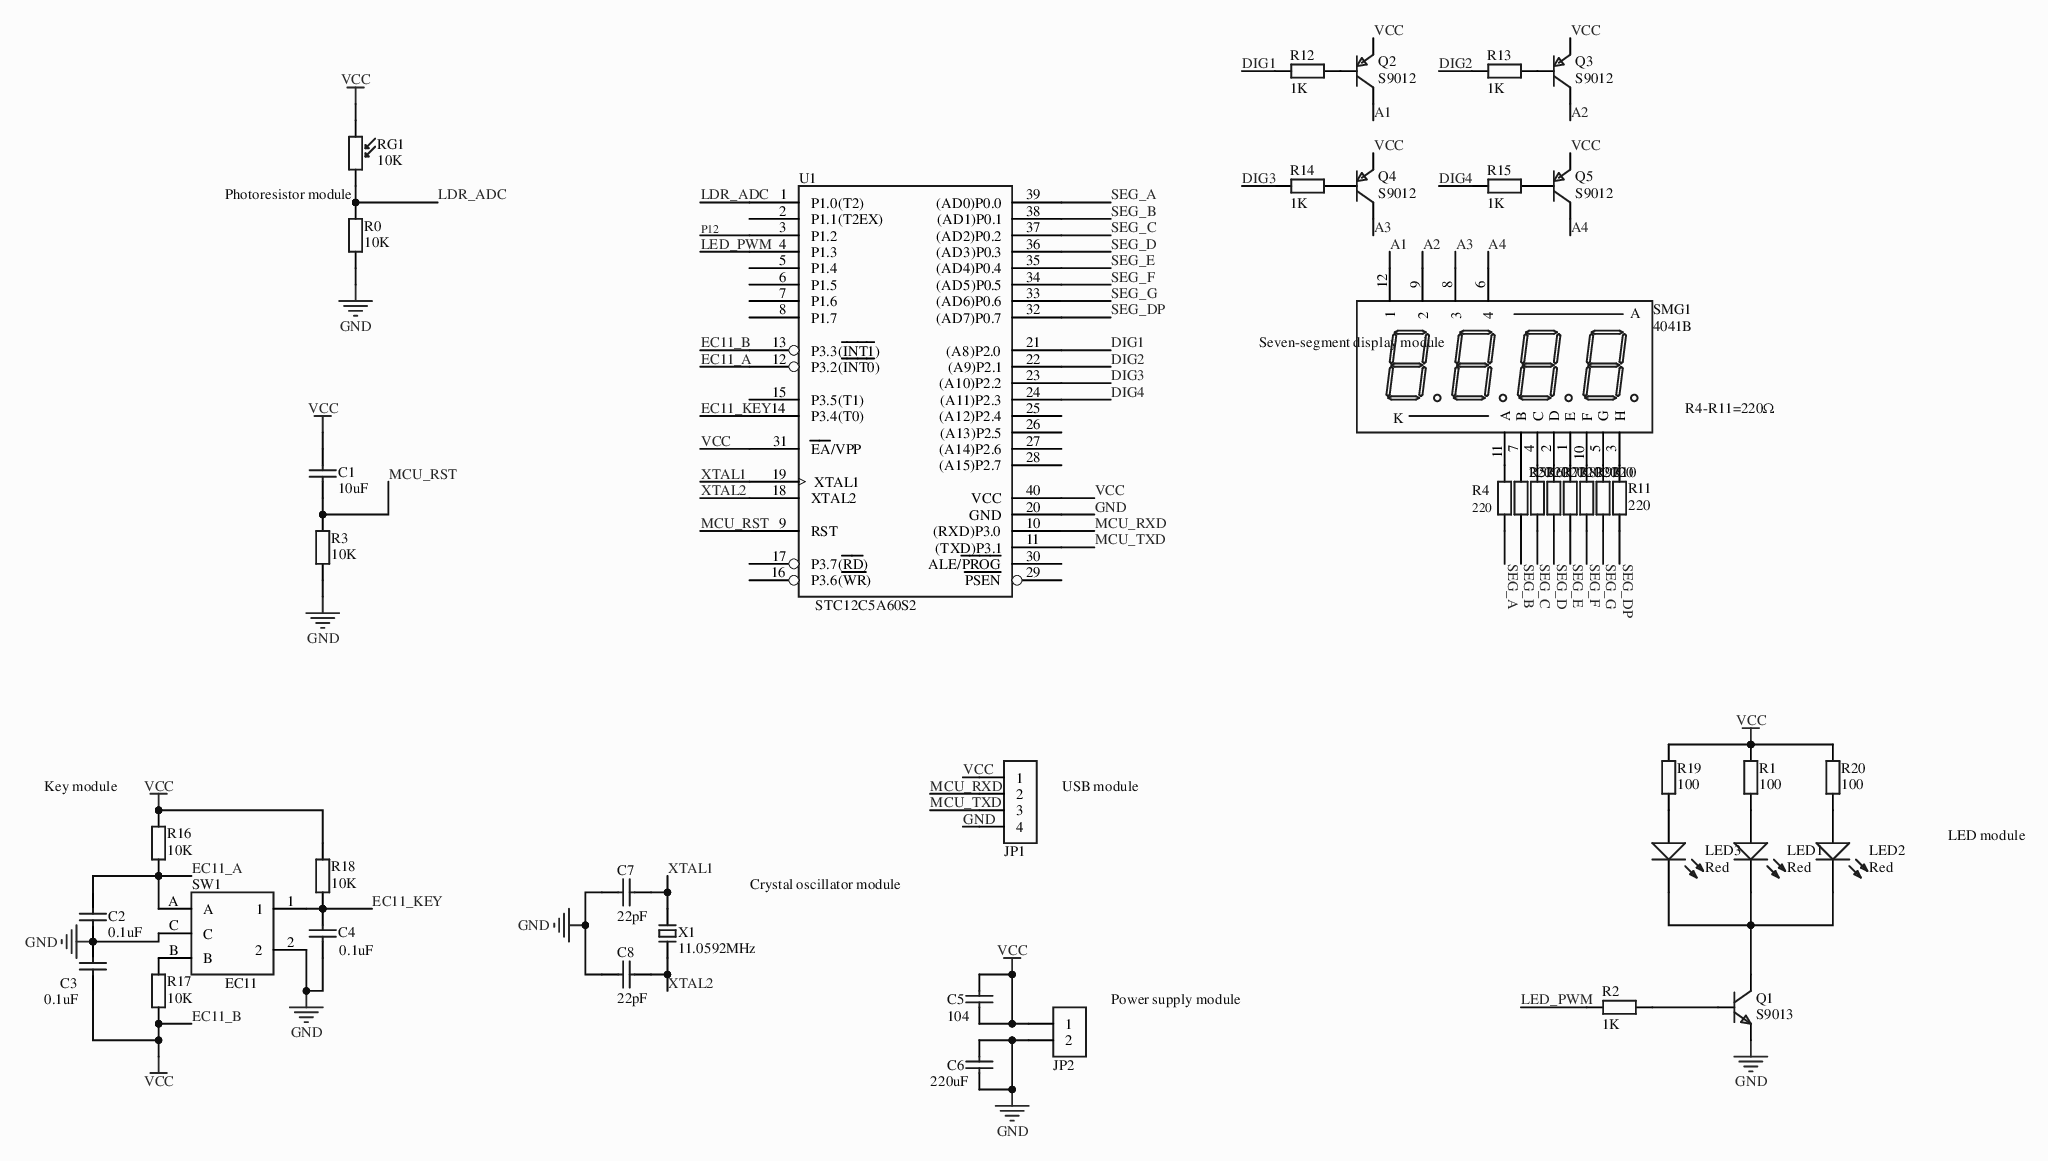
[diagram p0: MISC51984-3.schdoc]
# Altium project MISC51984-2.PrjPcb
1 sheet, 44 parts. Net scope: global (net labels, ports and power ports of the same name join across sheets).
Board file: MISC51984.pcbdoc

## Sheet MISC51984-3.schdoc
size 381 x 241 mm; SheetNumber: 1; SheetTotal: 1; Name: MISC51984

### Parts
C1  10uF  [C0805_L]
C2  0.1uF  [C0805_L]
C3  0.1uF  [C0805_L]
C4  0.1uF  [C0805_L]
C5  104  [CC 1.8*3.6]
C6  220uF  [C0805_L]
C7  22pF  [CC 1.8*3.6]
C8  22pF  [CC 1.8*3.6]
JP1  HDR-1X4  [XH2.54-LI-4P]  (value not drawn)
JP2  HDR-1X2  [XH2.54-LI-2P]  (value not drawn)
LED1  Red  [LED 3MM-B]
LED2  Red  [LED 3MM-B]
LED3  Red  [LED 3MM-B]
Q1  S9013  [TO92A]
Q2  S9012  [TO92A]
Q3  S9012  [TO92A]
Q4  S9012  [TO92A]
Q5  S9012  [TO92A]
R0  10K  [AXIAL0.4-1/4W]
R1  100  [AXIAL0.3-1/8W]
R2  1K  [AXIAL0.3-1/8W]
R3  10K  [AXIAL0.4-1/4W]
R4  220  [AXIAL0.4-1/4W]
R5  220  [AXIAL0.4-1/4W]
R6  220  [AXIAL0.4-1/4W]
R7  220  [AXIAL0.4-1/4W]
R8  220  [AXIAL0.4-1/4W]
R9  220  [AXIAL0.4-1/4W]
R10  220  [AXIAL0.4-1/4W]
R11  220  [AXIAL0.4-1/4W]
R12  1K  [AXIAL0.4-1/4W]
R13  1K  [AXIAL0.4-1/4W]
R14  1K  [AXIAL0.4-1/4W]
R15  1K  [AXIAL0.4-1/4W]
R16  10K  [AXIAL0.4-1/4W]
R17  10K  [AXIAL0.4-1/4W]
R18  10K  [AXIAL0.4-1/4W]
R19  100  [AXIAL0.3-1/8W]
R20  100  [AXIAL0.3-1/8W]
RG1  10K  [RG5528]
SMG1  4041B  [SMG 0.4-4P]
SW1  EC11  [EC11-B]
U1  STC12C5A60S2  [DIP-40]
X1  11.0592MHz  [HC-49S]

### Nets
VCC: C1.2 C3.1 C5.1 C5.2 JP1.1 JP2.1 Q2.1(E) Q3.1(E) Q4.1(E) Q5.1(E) R1.2 R16.2 R17.1 R18.2 R19.2 R20.2 RG1.1 U1.13(P3.3(~{INT1})) U1.31(~{EA}/VPP) U1.40(VCC)  [also labelled EC11_B]
GND: C2.1 C3.2 C4.1 C6.1 C6.2 C7.1 C8.1 JP1.4 JP2.2 Q1.1(E) R0.2 R3.2 SW1.2 SW1.C U1.20(GND)
A1: Q2.3(C) SMG1.12(1)
A2: Q3.3(C) SMG1.9(2)
A3: Q4.3(C) SMG1.8(3)
A4: Q5.3(C) SMG1.6(4)
DIG1: R12.1 U1.21((A8)P2.0)
DIG2: R13.1 U1.22((A9)P2.1)
DIG3: R14.1 U1.23((A10)P2.2)
DIG4: R15.1 U1.24((A11)P2.3)
EC11_A: C2.2 R16.1 SW1.A U1.12(P3.2(~{INT0}))
EC11_KEY: C4.2 R18.1 SW1.1 U1.14(P3.4(T0))
LDR_ADC: R0.1 RG1.2 U1.1(P1.0(T2))
LED_PWM: R2.1 U1.4(P1.3)
MCU_RST: C1.1 R3.1 U1.9(RST)
MCU_RXD: JP1.2 U1.10((RXD)P3.0)
MCU_TXD: JP1.3 U1.11((TXD)P3.1)
P12: U1.3(P1.2)
SEG_A: R4.2 U1.39((AD0)P0.0)
SEG_B: R5.1 U1.38((AD1)P0.1)
SEG_C: R6.1 U1.37((AD2)P0.2)
SEG_D: R7.1 U1.36((AD3)P0.3)
SEG_DP: R11.1 U1.32((AD7)P0.7)
SEG_E: R8.1 U1.35((AD4)P0.4)
SEG_F: R9.1 U1.34((AD5)P0.5)
SEG_G: R10.2 U1.33((AD6)P0.6)
XTAL1: C7.2 U1.19(XTAL1) X1.2
XTAL2: C8.2 U1.18(XTAL2) X1.1
NetLED1_1: LED1.1(A) R1.1
NetLED1_2: LED1.2(K) LED2.2(K) LED3.2(K) Q1.3(C)
NetLED2_1: LED2.1(A) R20.1
NetLED3_1: LED3.1(A) R19.1
NetQ1_2: Q1.2(B) R2.2
NetQ2_2: Q2.2(B) R12.2
NetQ3_2: Q3.2(B) R13.2
NetQ4_2: Q4.2(B) R14.2
NetQ5_2: Q5.2(B) R15.2
NetR4_1: R4.1 SMG1.11(A)
NetR5_2: R5.2 SMG1.7(B)
NetR6_2: R6.2 SMG1.4(C)
NetR7_2: R7.2 SMG1.2(D)
NetR8_2: R8.2 SMG1.1(E)
NetR9_2: R9.2 SMG1.10(F)
NetR10_1: R10.1 SMG1.5(G)
NetR11_2: R11.2 SMG1.3(H)
NetR17_2: R17.2 SW1.B

Not connected (* = marked no-connect by the designer): U1 2(P1.1(T2EX)) 5(P1.4) 6(P1.5) 7(P1.6) 8(P1.7) 15(P3.5(T1)) 16(P3.6(~{WR})) 17(P3.7(~{RD})) 25((A12)P2.4) 26((A13)P2.5) 27((A14)P2.6) 28((A15)P2.7) 29(~{PSEN}) 30(ALE/~{PROG})

### Notes on the sheet
- Photoresistor module
- (near SMG1) Seven-segment display module
- R4-R11=220Ω
- (near R16) Key module
- (near JP1) USB module
- LED module
- Crystal oscillator module
- (near JP2) Power supply module

### Library data of the parts
C1 = 10uF: SMD capacitor/MLCC; BOM名称: Non-polar SMD capacitor; 当前库版本V2022.12.25 @: 最新版本发布; Origin Footprint: C0201_L; OriginFootprint 2: C0402_L; OriginFootprint 3: C0603_L; OriginFootprint 4: C1206_L; OriginFootprint 5: C1210_L; OriginFootprint 6: C1808_L; OriginFootprint 7: C1812_L; OriginFootprint 8: C1825_L; OriginFootprint 9: C2225_L; OriginFootprint 10: C0201_M; OriginFootprint 11: C0402_M; OriginFootprint 12: C0603_M; OriginFootprint 13: C0805_M; OriginFootprint 14: C1206_M; OriginFootprint 15: C1210_M; OriginFootprint 16: C1808_M; OriginFootprint 17: C1812_M; OriginFootprint 18: C1825_M; OriginFootprint 19: C2225_M; OriginFootprint 20: C0201_NS; OriginFootprint 21: C0402_NS; OriginFootprint 22: C01005_NS; OriginFootprint 23: C0805_NS; OriginFootprint 24: C1206_NS; OriginFootprint 25: C1210_NS; OriginFootprint 26: C0603_NS; OriginFootprint 27: C0204_NS; OriginFootprint 28: C1111_NS; OriginFootprint 29: C2220; OriginFootprint 30: C3838; UniqueId: 5fb4f22ffcb6a001; SymbolName: C; AddInBom: yes; OriginModelName: C0805H13-2S; Device: 10uF; DesignItemID: C; LibraryName: 0.1 - Resistor-Capacitor-Inductor-Fuse-Crystal oscillator-Crystal-Ferrite bead-Potentiometer-Supercapacitor-Feedthrough capacitor; FootprintName: C0805_L
C2 = 0.1uF: SMD capacitor/MLCC; BOM名称: Non-polar SMD capacitor; 当前库版本V2022.12.25 @: 最新版本发布; Origin Footprint: C0201_L; OriginFootprint 2: C0402_L; OriginFootprint 3: C0603_L; OriginFootprint 4: C1206_L; OriginFootprint 5: C1210_L; OriginFootprint 6: C1808_L; OriginFootprint 7: C1812_L; OriginFootprint 8: C1825_L; OriginFootprint 9: C2225_L; OriginFootprint 10: C0201_M; OriginFootprint 11: C0402_M; OriginFootprint 12: C0603_M; OriginFootprint 13: C0805_M; OriginFootprint 14: C1206_M; OriginFootprint 15: C1210_M; OriginFootprint 16: C1808_M; OriginFootprint 17: C1812_M; OriginFootprint 18: C1825_M; OriginFootprint 19: C2225_M; OriginFootprint 20: C0201_NS; OriginFootprint 21: C0402_NS; OriginFootprint 22: C01005_NS; OriginFootprint 23: C0805_NS; OriginFootprint 24: C1206_NS; OriginFootprint 25: C1210_NS; OriginFootprint 26: C0603_NS; OriginFootprint 27: C0204_NS; OriginFootprint 28: C1111_NS; OriginFootprint 29: C2220; OriginFootprint 30: C3838; UniqueId: 21d50210554cb61f; SymbolName: C; AddInBom: yes; OriginModelName: C0805H13-2S; Device: 0.1uF; DesignItemID: C; LibraryName: 0.1 - Resistor-Capacitor-Inductor-Fuse-Crystal oscillator-Crystal-Ferrite bead-Potentiometer-Supercapacitor-Feedthrough capacitor; FootprintName: C0805_L
C3 = 0.1uF: SMD capacitor/MLCC; BOM名称: Non-polar SMD capacitor; 当前库版本V2022.12.25 @: 最新版本发布; Origin Footprint: C0201_L; OriginFootprint 2: C0402_L; OriginFootprint 3: C0603_L; OriginFootprint 4: C1206_L; OriginFootprint 5: C1210_L; OriginFootprint 6: C1808_L; OriginFootprint 7: C1812_L; OriginFootprint 8: C1825_L; OriginFootprint 9: C2225_L; OriginFootprint 10: C0201_M; OriginFootprint 11: C0402_M; OriginFootprint 12: C0603_M; OriginFootprint 13: C0805_M; OriginFootprint 14: C1206_M; OriginFootprint 15: C1210_M; OriginFootprint 16: C1808_M; OriginFootprint 17: C1812_M; OriginFootprint 18: C1825_M; OriginFootprint 19: C2225_M; OriginFootprint 20: C0201_NS; OriginFootprint 21: C0402_NS; OriginFootprint 22: C01005_NS; OriginFootprint 23: C0805_NS; OriginFootprint 24: C1206_NS; OriginFootprint 25: C1210_NS; OriginFootprint 26: C0603_NS; OriginFootprint 27: C0204_NS; OriginFootprint 28: C1111_NS; OriginFootprint 29: C2220; OriginFootprint 30: C3838; UniqueId: ec64484c8c07847f; SymbolName: C; AddInBom: yes; OriginModelName: C0805H13-2S; Device: 0.1uF; DesignItemID: C; LibraryName: 0.1 - Resistor-Capacitor-Inductor-Fuse-Crystal oscillator-Crystal-Ferrite bead-Potentiometer-Supercapacitor-Feedthrough capacitor; FootprintName: C0805_L
C4 = 0.1uF: SMD capacitor/MLCC; BOM名称: Non-polar SMD capacitor; 当前库版本V2022.12.25 @: 最新版本发布; Origin Footprint: C0201_L; OriginFootprint 2: C0402_L; OriginFootprint 3: C0603_L; OriginFootprint 4: C1206_L; OriginFootprint 5: C1210_L; OriginFootprint 6: C1808_L; OriginFootprint 7: C1812_L; OriginFootprint 8: C1825_L; OriginFootprint 9: C2225_L; OriginFootprint 10: C0201_M; OriginFootprint 11: C0402_M; OriginFootprint 12: C0603_M; OriginFootprint 13: C0805_M; OriginFootprint 14: C1206_M; OriginFootprint 15: C1210_M; OriginFootprint 16: C1808_M; OriginFootprint 17: C1812_M; OriginFootprint 18: C1825_M; OriginFootprint 19: C2225_M; OriginFootprint 20: C0201_NS; OriginFootprint 21: C0402_NS; OriginFootprint 22: C01005_NS; OriginFootprint 23: C0805_NS; OriginFootprint 24: C1206_NS; OriginFootprint 25: C1210_NS; OriginFootprint 26: C0603_NS; OriginFootprint 27: C0204_NS; OriginFootprint 28: C1111_NS; OriginFootprint 29: C2220; OriginFootprint 30: C3838; UniqueId: 623e2bb2442f04df; SymbolName: C; AddInBom: yes; OriginModelName: C0805H13-2S; Device: 0.1uF; DesignItemID: C; LibraryName: 0.1 - Resistor-Capacitor-Inductor-Fuse-Crystal oscillator-Crystal-Ferrite bead-Potentiometer-Supercapacitor-Feedthrough capacitor; FootprintName: C0805_L
C5 = 104: Ceramic capacitor; BOM名称: Through-hole ceramic capacitor; 当前库版本V2022.12.25 @: 最新版本发布; Origin Footprint: CC 2.2*5; UniqueId: 05d417a4d81547fc; SymbolName: CC; AddInBom: yes; OriginModelName: CC_1.8x3.6-2; Device: 104; DesignItemID: CC; LibraryName: 0.1 - Resistor-Capacitor-Inductor-Fuse-Crystal oscillator-Crystal-Ferrite bead-Potentiometer-Supercapacitor-Feedthrough capacitor; FootprintName: CC 1.8*3.6
C6 = 220uF: SMD capacitor/MLCC; BOM名称: Non-polar SMD capacitor; 当前库版本V2022.12.25 @: 最新版本发布; Origin Footprint: C0201_L; OriginFootprint 2: C0402_L; OriginFootprint 3: C0603_L; OriginFootprint 4: C1206_L; OriginFootprint 5: C1210_L; OriginFootprint 6: C1808_L; OriginFootprint 7: C1812_L; OriginFootprint 8: C1825_L; OriginFootprint 9: C2225_L; OriginFootprint 10: C0201_M; OriginFootprint 11: C0402_M; OriginFootprint 12: C0603_M; OriginFootprint 13: C0805_M; OriginFootprint 14: C1206_M; OriginFootprint 15: C1210_M; OriginFootprint 16: C1808_M; OriginFootprint 17: C1812_M; OriginFootprint 18: C1825_M; OriginFootprint 19: C2225_M; OriginFootprint 20: C0201_NS; OriginFootprint 21: C0402_NS; OriginFootprint 22: C01005_NS; OriginFootprint 23: C0805_NS; OriginFootprint 24: C1206_NS; OriginFootprint 25: C1210_NS; OriginFootprint 26: C0603_NS; OriginFootprint 27: C0204_NS; OriginFootprint 28: C1111_NS; OriginFootprint 29: C2220; OriginFootprint 30: C3838; UniqueId: d45ffe04e43665a4; SymbolName: C; AddInBom: yes; OriginModelName: C0805H13-2S; Device: 220uF; DesignItemID: C; LibraryName: 0.1 - Resistor-Capacitor-Inductor-Fuse-Crystal oscillator-Crystal-Ferrite bead-Potentiometer-Supercapacitor-Feedthrough capacitor; FootprintName: C0805_L
C7 = 22pF: Ceramic capacitor; BOM名称: Through-hole ceramic capacitor; 当前库版本V2022.12.25 @: 最新版本发布; Origin Footprint: CC 2.2*5; UniqueId: 3007ca2539a35480; SymbolName: CC; AddInBom: yes; OriginModelName: CC_1.8x3.6-2; Device: 22pF; DesignItemID: CC; LibraryName: 0.1 - Resistor-Capacitor-Inductor-Fuse-Crystal oscillator-Crystal-Ferrite bead-Potentiometer-Supercapacitor-Feedthrough capacitor; FootprintName: CC 1.8*3.6
C8 = 22pF: Ceramic capacitor; BOM名称: Through-hole ceramic capacitor; 当前库版本V2022.12.25 @: 最新版本发布; Origin Footprint: CC 2.2*5; UniqueId: 878ab3ab0cce2757; SymbolName: CC; AddInBom: yes; OriginModelName: CC_1.8x3.6-2; Device: 22pF; DesignItemID: CC; LibraryName: 0.1 - Resistor-Capacitor-Inductor-Fuse-Crystal oscillator-Crystal-Ferrite bead-Potentiometer-Supercapacitor-Feedthrough capacitor; FootprintName: CC 1.8*3.6
JP1 = HDR-1X4: 4P connector; Origin Footprint: XH2.54-W-4P; OriginFootprint 2: HDR2.54-LI-4P; OriginFootprint 3: HDR2.54-M-LI-4P; OriginFootprint 4: HDR2.54-WI-4P; OriginFootprint 5: HDR2.54-WS-4P; OriginFootprint 6: HDR2.54-Y-LI-4P; OriginFootprint 7: HDR2.54-M-WT-4P; OriginFootprint 8: KF2510-LI-4P; OriginFootprint 9: XH2.54-WT-4P; OriginFootprint 10: XH2.54-LS-4P; OriginFootprint 11: KF2EDGK-2.54-LI-4P; OriginFootprint 12: KF2EDGK-2.54-WI-4P; UniqueId: 3f7cd319db4ef0a6; SymbolName: Header 4; AddInBom: yes; OriginModelName: XH2_54-4P; Device: HDR-1X4; BOM名称: 4P connector; DesignItemID: Header 4; LibraryName: 5.5 - 2.54mm connectors (KF2EDGK_XH2.54_2.54 pin header/socket); FootprintName: XH2.54-LI-4P
JP2 = HDR-1X2: 2P connector; Origin Footprint: XH2.54-W-2P; OriginFootprint 2: HDR2.54-LI-2P; OriginFootprint 3: HDR2.54-M-LI-2P; OriginFootprint 4: HDR2.54-WI-2P; OriginFootprint 5: HDR2.54-WS-2P; OriginFootprint 6: HDR2.54-Y-LI-2P; OriginFootprint 7: HDR2.54-M-WT-2P; OriginFootprint 8: KF2510-LI-2P; OriginFootprint 9: XH2.54-WT-2P; OriginFootprint 10: XH2.54-LS-2P; OriginFootprint 11: KF2EDGK-2.54-LI-2P; OriginFootprint 12: KF2EDGK-2.54-WI-2P; UniqueId: e68233645d205bf0; SymbolName: Header 2; AddInBom: yes; OriginModelName: XH2_54-2P; Device: HDR-1X2; BOM名称: 2P connector; DesignItemID: Header 2; LibraryName: 5.5 - 2.54mm connectors (KF2EDGK_XH2.54_2.54 pin header/socket); FootprintName: XH2.54-LI-2P
LED1 = 红色: 3mm through-hole LED; BOM名称: Plug-in LED; Origin Footprint: LED 3MM-G; OriginFootprint 2: LED 3MM-R; OriginFootprint 3: LED 3MM-Y; OriginFootprint 4: LED 3MM-YC; OriginFootprint 5: LED 3MM-W; OriginFootprint 6: LED 3MM-G-H; OriginFootprint 7: LED 3MM-R-H; OriginFootprint 8: LED 3MM-Y-H; UniqueId: a4c4b307afb8d999; SymbolName: LED-3MM; AddInBom: yes; OriginModelName: LED_3MM-B; Device: Red; DesignItemID: LED-3MM; LibraryName: 0.3 - LED-IR diode_receiver tube-Optocoupler; FootprintName: LED 3MM-B
LED2 = 红色: 3mm through-hole LED; BOM名称: Plug-in LED; Origin Footprint: LED 3MM-G; OriginFootprint 2: LED 3MM-R; OriginFootprint 3: LED 3MM-Y; OriginFootprint 4: LED 3MM-YC; OriginFootprint 5: LED 3MM-W; OriginFootprint 6: LED 3MM-G-H; OriginFootprint 7: LED 3MM-R-H; OriginFootprint 8: LED 3MM-Y-H; UniqueId: a245eb2d2aad9559; SymbolName: LED-3MM; AddInBom: yes; OriginModelName: LED_3MM-B; Device: Red; DesignItemID: LED-3MM; LibraryName: 0.3 - LED-IR diode_receiver tube-Optocoupler; FootprintName: LED 3MM-B
LED3 = 红色: 3mm through-hole LED; BOM名称: Plug-in LED; Origin Footprint: LED 3MM-G; OriginFootprint 2: LED 3MM-R; OriginFootprint 3: LED 3MM-Y; OriginFootprint 4: LED 3MM-YC; OriginFootprint 5: LED 3MM-W; OriginFootprint 6: LED 3MM-G-H; OriginFootprint 7: LED 3MM-R-H; OriginFootprint 8: LED 3MM-Y-H; UniqueId: 01e448f2d6732d04; SymbolName: LED-3MM; AddInBom: yes; OriginModelName: LED_3MM-B; Device: Red; DesignItemID: LED-3MM; LibraryName: 0.3 - LED-IR diode_receiver tube-Optocoupler; FootprintName: LED 3MM-B
Q1 = S9013: Low-frequency amplifier, NPN type; 参数: 50V 0.5A 0.625W; Origin Footprint: TO92B; UniqueId: 047b734180970fea; SymbolName: 9013-DIP; AddInBom: yes; Device: S9013; BOM名称: Low-frequency amplifier, NPN type; DesignItemID: 9013-DIP; LibraryName: 0.4 - Transistors-FETs-Thyristors; FootprintName: TO92A; OriginModelName: TO92A
Q2 = S9012: Low-frequency amplifier, PNP type; 参数: 50V 0.5A 0.625W; Origin Footprint: TO92B; UniqueId: 4adba29ee04e5395; SymbolName: 9012-DIP; AddInBom: yes; Device: S9012; BOM名称: Low-frequency amplifier, PNP type; DesignItemID: 9012-DIP; LibraryName: 0.4 - Transistors-FETs-Thyristors; FootprintName: TO92A; OriginModelName: TO92A
Q3 = S9012: Low-frequency amplifier, PNP type; 参数: 50V 0.5A 0.625W; Origin Footprint: TO92B; UniqueId: 44595dc3afca5345; SymbolName: 9012-DIP; AddInBom: yes; Device: S9012; BOM名称: Low-frequency amplifier, PNP type; DesignItemID: 9012-DIP; LibraryName: 0.4 - Transistors-FETs-Thyristors; FootprintName: TO92A; OriginModelName: TO92A
Q4 = S9012: Low-frequency amplifier, PNP type; 参数: 50V 0.5A 0.625W; Origin Footprint: TO92B; UniqueId: 3881765f76976367; SymbolName: 9012-DIP; AddInBom: yes; Device: S9012; BOM名称: Low-frequency amplifier, PNP type; DesignItemID: 9012-DIP; LibraryName: 0.4 - Transistors-FETs-Thyristors; FootprintName: TO92A; OriginModelName: TO92A
Q5 = S9012: Low-frequency amplifier, PNP type; 参数: 50V 0.5A 0.625W; Origin Footprint: TO92B; UniqueId: 29f2ccd72f89748e; SymbolName: 9012-DIP; AddInBom: yes; Device: S9012; BOM名称: Low-frequency amplifier, PNP type; DesignItemID: 9012-DIP; LibraryName: 0.4 - Transistors-FETs-Thyristors; FootprintName: TO92A; OriginModelName: TO92A
R0 = 10K_1: SMD resistor; Origin Footprint: R0201_L; OriginFootprint 2: R0402_L; OriginFootprint 3: R0603_L; OriginFootprint 4: R0805_L; OriginFootprint 5: R1206_L; OriginFootprint 6: R1210_L; OriginFootprint 7: R1812_L; OriginFootprint 8: R2010_L; OriginFootprint 9: R2512_L; OriginFootprint 10: R0201_M; OriginFootprint 11: R0402_M; OriginFootprint 12: R0603_M; OriginFootprint 13: R0805_M; OriginFootprint 14: R1206_M; OriginFootprint 15: R1210_M; OriginFootprint 16: R1812_M; OriginFootprint 17: R2010_M; OriginFootprint 18: R2512_M; OriginFootprint 19: R0201_NS; OriginFootprint 20: R0402_NS; OriginFootprint 21: R01005_NS; OriginFootprint 22: R0603_NS; OriginFootprint 23: R0805_NS; OriginFootprint 24: R1206_NS; OriginFootprint 25: R1210_NS; UniqueId: ac6f166285f3c9f2; SymbolName: R; AddInBom: yes; OriginModelName: rs_1-4w; Device: 10K_1; BOM名称: SMD resistor; DesignItemID: R; LibraryName: 0.1 - Resistor-Capacitor-Inductor-Fuse-Crystal oscillator-Crystal-Ferrite bead-Potentiometer-Supercapacitor-Feedthrough capacitor; FootprintName: AXIAL0.4-1/4W
R1 = 100: SMD resistor; Origin Footprint: R0201_L; OriginFootprint 2: R0402_L; OriginFootprint 3: R0603_L; OriginFootprint 4: R0805_L; OriginFootprint 5: R1206_L; OriginFootprint 6: R1210_L; OriginFootprint 7: R1812_L; OriginFootprint 8: R2010_L; OriginFootprint 9: R2512_L; OriginFootprint 10: R0201_M; OriginFootprint 11: R0402_M; OriginFootprint 12: R0603_M; OriginFootprint 13: R0805_M; OriginFootprint 14: R1206_M; OriginFootprint 15: R1210_M; OriginFootprint 16: R1812_M; OriginFootprint 17: R2010_M; OriginFootprint 18: R2512_M; OriginFootprint 19: R0201_NS; OriginFootprint 20: R0402_NS; OriginFootprint 21: R01005_NS; OriginFootprint 22: R0603_NS; OriginFootprint 23: R0805_NS; OriginFootprint 24: R1206_NS; OriginFootprint 25: R1210_NS; UniqueId: 4e166b190d4de1c3; SymbolName: R; AddInBom: yes; OriginModelName: rs_1-8w; Device: 100; BOM名称: SMD resistor; DesignItemID: R; LibraryName: 0.1 - Resistor-Capacitor-Inductor-Fuse-Crystal oscillator-Crystal-Ferrite bead-Potentiometer-Supercapacitor-Feedthrough capacitor; FootprintName: AXIAL0.3-1/8W
R2 = 1K: SMD resistor; Origin Footprint: R0201_L; OriginFootprint 2: R0402_L; OriginFootprint 3: R0603_L; OriginFootprint 4: R0805_L; OriginFootprint 5: R1206_L; OriginFootprint 6: R1210_L; OriginFootprint 7: R1812_L; OriginFootprint 8: R2010_L; OriginFootprint 9: R2512_L; OriginFootprint 10: R0201_M; OriginFootprint 11: R0402_M; OriginFootprint 12: R0603_M; OriginFootprint 13: R0805_M; OriginFootprint 14: R1206_M; OriginFootprint 15: R1210_M; OriginFootprint 16: R1812_M; OriginFootprint 17: R2010_M; OriginFootprint 18: R2512_M; OriginFootprint 19: R0201_NS; OriginFootprint 20: R0402_NS; OriginFootprint 21: R01005_NS; OriginFootprint 22: R0603_NS; OriginFootprint 23: R0805_NS; OriginFootprint 24: R1206_NS; OriginFootprint 25: R1210_NS; UniqueId: 06442d24ab060343; SymbolName: R; AddInBom: yes; OriginModelName: rs_1-8w; Device: 1K; BOM名称: SMD resistor; DesignItemID: R; LibraryName: 0.1 - Resistor-Capacitor-Inductor-Fuse-Crystal oscillator-Crystal-Ferrite bead-Potentiometer-Supercapacitor-Feedthrough capacitor; FootprintName: AXIAL0.3-1/8W
R3 = 10K_1: SMD resistor; Origin Footprint: R0201_L; OriginFootprint 2: R0402_L; OriginFootprint 3: R0603_L; OriginFootprint 4: R0805_L; OriginFootprint 5: R1206_L; OriginFootprint 6: R1210_L; OriginFootprint 7: R1812_L; OriginFootprint 8: R2010_L; OriginFootprint 9: R2512_L; OriginFootprint 10: R0201_M; OriginFootprint 11: R0402_M; OriginFootprint 12: R0603_M; OriginFootprint 13: R0805_M; OriginFootprint 14: R1206_M; OriginFootprint 15: R1210_M; OriginFootprint 16: R1812_M; OriginFootprint 17: R2010_M; OriginFootprint 18: R2512_M; OriginFootprint 19: R0201_NS; OriginFootprint 20: R0402_NS; OriginFootprint 21: R01005_NS; OriginFootprint 22: R0603_NS; OriginFootprint 23: R0805_NS; OriginFootprint 24: R1206_NS; OriginFootprint 25: R1210_NS; UniqueId: 6e26aea592918673; SymbolName: R; AddInBom: yes; OriginModelName: rs_1-4w; Device: 10K_1; BOM名称: SMD resistor; OriginFootprint 26: AXIAL0.4-1/4W; DesignItemID: R; LibraryName: 0.1 - Resistor-Capacitor-Inductor-Fuse-Crystal oscillator-Crystal-Ferrite bead-Potentiometer-Supercapacitor-Feedthrough capacitor; FootprintName: AXIAL0.4-1/4W
R4 = 220: SMD resistor; Origin Footprint: R0201_L; OriginFootprint 2: R0402_L; OriginFootprint 3: R0603_L; OriginFootprint 4: R0805_L; OriginFootprint 5: R1206_L; OriginFootprint 6: R1210_L; OriginFootprint 7: R1812_L; OriginFootprint 8: R2010_L; OriginFootprint 9: R2512_L; OriginFootprint 10: R0201_M; OriginFootprint 11: R0402_M; OriginFootprint 12: R0603_M; OriginFootprint 13: R0805_M; OriginFootprint 14: R1206_M; OriginFootprint 15: R1210_M; OriginFootprint 16: R1812_M; OriginFootprint 17: R2010_M; OriginFootprint 18: R2512_M; OriginFootprint 19: R0201_NS; OriginFootprint 20: R0402_NS; OriginFootprint 21: R01005_NS; OriginFootprint 22: R0603_NS; OriginFootprint 23: R0805_NS; OriginFootprint 24: R1206_NS; OriginFootprint 25: R1210_NS; UniqueId: 49359f7360e76581; SymbolName: R; AddInBom: yes; OriginModelName: rs_1-4w; Device: 220; BOM名称: SMD resistor; DesignItemID: R; LibraryName: 0.1 - Resistor-Capacitor-Inductor-Fuse-Crystal oscillator-Crystal-Ferrite bead-Potentiometer-Supercapacitor-Feedthrough capacitor; FootprintName: AXIAL0.4-1/4W
R5 = 220: SMD resistor; Origin Footprint: R0201_L; OriginFootprint 2: R0402_L; OriginFootprint 3: R0603_L; OriginFootprint 4: R0805_L; OriginFootprint 5: R1206_L; OriginFootprint 6: R1210_L; OriginFootprint 7: R1812_L; OriginFootprint 8: R2010_L; OriginFootprint 9: R2512_L; OriginFootprint 10: R0201_M; OriginFootprint 11: R0402_M; OriginFootprint 12: R0603_M; OriginFootprint 13: R0805_M; OriginFootprint 14: R1206_M; OriginFootprint 15: R1210_M; OriginFootprint 16: R1812_M; OriginFootprint 17: R2010_M; OriginFootprint 18: R2512_M; OriginFootprint 19: R0201_NS; OriginFootprint 20: R0402_NS; OriginFootprint 21: R01005_NS; OriginFootprint 22: R0603_NS; OriginFootprint 23: R0805_NS; OriginFootprint 24: R1206_NS; OriginFootprint 25: R1210_NS; UniqueId: 96bd3269827a783e; SymbolName: R; AddInBom: yes; OriginModelName: rs_1-4w; Device: 220; BOM名称: SMD resistor; DesignItemID: R; LibraryName: 0.1 - Resistor-Capacitor-Inductor-Fuse-Crystal oscillator-Crystal-Ferrite bead-Potentiometer-Supercapacitor-Feedthrough capacitor; FootprintName: AXIAL0.4-1/4W
R6 = 220: SMD resistor; Origin Footprint: R0201_L; OriginFootprint 2: R0402_L; OriginFootprint 3: R0603_L; OriginFootprint 4: R0805_L; OriginFootprint 5: R1206_L; OriginFootprint 6: R1210_L; OriginFootprint 7: R1812_L; OriginFootprint 8: R2010_L; OriginFootprint 9: R2512_L; OriginFootprint 10: R0201_M; OriginFootprint 11: R0402_M; OriginFootprint 12: R0603_M; OriginFootprint 13: R0805_M; OriginFootprint 14: R1206_M; OriginFootprint 15: R1210_M; OriginFootprint 16: R1812_M; OriginFootprint 17: R2010_M; OriginFootprint 18: R2512_M; OriginFootprint 19: R0201_NS; OriginFootprint 20: R0402_NS; OriginFootprint 21: R01005_NS; OriginFootprint 22: R0603_NS; OriginFootprint 23: R0805_NS; OriginFootprint 24: R1206_NS; OriginFootprint 25: R1210_NS; UniqueId: c9a24d22ca7022dc; SymbolName: R; AddInBom: yes; OriginModelName: rs_1-4w; Device: 220; BOM名称: SMD resistor; DesignItemID: R; LibraryName: 0.1 - Resistor-Capacitor-Inductor-Fuse-Crystal oscillator-Crystal-Ferrite bead-Potentiometer-Supercapacitor-Feedthrough capacitor; FootprintName: AXIAL0.4-1/4W
R7 = 220: SMD resistor; Origin Footprint: R0201_L; OriginFootprint 2: R0402_L; OriginFootprint 3: R0603_L; OriginFootprint 4: R0805_L; OriginFootprint 5: R1206_L; OriginFootprint 6: R1210_L; OriginFootprint 7: R1812_L; OriginFootprint 8: R2010_L; OriginFootprint 9: R2512_L; OriginFootprint 10: R0201_M; OriginFootprint 11: R0402_M; OriginFootprint 12: R0603_M; OriginFootprint 13: R0805_M; OriginFootprint 14: R1206_M; OriginFootprint 15: R1210_M; OriginFootprint 16: R1812_M; OriginFootprint 17: R2010_M; OriginFootprint 18: R2512_M; OriginFootprint 19: R0201_NS; OriginFootprint 20: R0402_NS; OriginFootprint 21: R01005_NS; OriginFootprint 22: R0603_NS; OriginFootprint 23: R0805_NS; OriginFootprint 24: R1206_NS; OriginFootprint 25: R1210_NS; UniqueId: 01f5c70ff2630ee7; SymbolName: R; AddInBom: yes; OriginModelName: rs_1-4w; Device: 220; BOM名称: SMD resistor; DesignItemID: R; LibraryName: 0.1 - Resistor-Capacitor-Inductor-Fuse-Crystal oscillator-Crystal-Ferrite bead-Potentiometer-Supercapacitor-Feedthrough capacitor; FootprintName: AXIAL0.4-1/4W
R8 = 220: SMD resistor; Origin Footprint: R0201_L; OriginFootprint 2: R0402_L; OriginFootprint 3: R0603_L; OriginFootprint 4: R0805_L; OriginFootprint 5: R1206_L; OriginFootprint 6: R1210_L; OriginFootprint 7: R1812_L; OriginFootprint 8: R2010_L; OriginFootprint 9: R2512_L; OriginFootprint 10: R0201_M; OriginFootprint 11: R0402_M; OriginFootprint 12: R0603_M; OriginFootprint 13: R0805_M; OriginFootprint 14: R1206_M; OriginFootprint 15: R1210_M; OriginFootprint 16: R1812_M; OriginFootprint 17: R2010_M; OriginFootprint 18: R2512_M; OriginFootprint 19: R0201_NS; OriginFootprint 20: R0402_NS; OriginFootprint 21: R01005_NS; OriginFootprint 22: R0603_NS; OriginFootprint 23: R0805_NS; OriginFootprint 24: R1206_NS; OriginFootprint 25: R1210_NS; UniqueId: f0665cc51e401020; SymbolName: R; AddInBom: yes; OriginModelName: rs_1-4w; Device: 220; BOM名称: SMD resistor; DesignItemID: R; LibraryName: 0.1 - Resistor-Capacitor-Inductor-Fuse-Crystal oscillator-Crystal-Ferrite bead-Potentiometer-Supercapacitor-Feedthrough capacitor; FootprintName: AXIAL0.4-1/4W
R9 = 220: SMD resistor; Origin Footprint: R0201_L; OriginFootprint 2: R0402_L; OriginFootprint 3: R0603_L; OriginFootprint 4: R0805_L; OriginFootprint 5: R1206_L; OriginFootprint 6: R1210_L; OriginFootprint 7: R1812_L; OriginFootprint 8: R2010_L; OriginFootprint 9: R2512_L; OriginFootprint 10: R0201_M; OriginFootprint 11: R0402_M; OriginFootprint 12: R0603_M; OriginFootprint 13: R0805_M; OriginFootprint 14: R1206_M; OriginFootprint 15: R1210_M; OriginFootprint 16: R1812_M; OriginFootprint 17: R2010_M; OriginFootprint 18: R2512_M; OriginFootprint 19: R0201_NS; OriginFootprint 20: R0402_NS; OriginFootprint 21: R01005_NS; OriginFootprint 22: R0603_NS; OriginFootprint 23: R0805_NS; OriginFootprint 24: R1206_NS; OriginFootprint 25: R1210_NS; UniqueId: 7a9d276dcc23a651; SymbolName: R; AddInBom: yes; OriginModelName: rs_1-4w; Device: 220; BOM名称: SMD resistor; DesignItemID: R; LibraryName: 0.1 - Resistor-Capacitor-Inductor-Fuse-Crystal oscillator-Crystal-Ferrite bead-Potentiometer-Supercapacitor-Feedthrough capacitor; FootprintName: AXIAL0.4-1/4W
R10 = 220: SMD resistor; Origin Footprint: R0201_L; OriginFootprint 2: R0402_L; OriginFootprint 3: R0603_L; OriginFootprint 4: R0805_L; OriginFootprint 5: R1206_L; OriginFootprint 6: R1210_L; OriginFootprint 7: R1812_L; OriginFootprint 8: R2010_L; OriginFootprint 9: R2512_L; OriginFootprint 10: R0201_M; OriginFootprint 11: R0402_M; OriginFootprint 12: R0603_M; OriginFootprint 13: R0805_M; OriginFootprint 14: R1206_M; OriginFootprint 15: R1210_M; OriginFootprint 16: R1812_M; OriginFootprint 17: R2010_M; OriginFootprint 18: R2512_M; OriginFootprint 19: R0201_NS; OriginFootprint 20: R0402_NS; OriginFootprint 21: R01005_NS; OriginFootprint 22: R0603_NS; OriginFootprint 23: R0805_NS; OriginFootprint 24: R1206_NS; OriginFootprint 25: R1210_NS; UniqueId: 7663007c1f2bc029; SymbolName: R; AddInBom: yes; OriginModelName: rs_1-4w; Device: 220; BOM名称: SMD resistor; DesignItemID: R; LibraryName: 0.1 - Resistor-Capacitor-Inductor-Fuse-Crystal oscillator-Crystal-Ferrite bead-Potentiometer-Supercapacitor-Feedthrough capacitor; FootprintName: AXIAL0.4-1/4W
R11 = 220: SMD resistor; Origin Footprint: R0201_L; OriginFootprint 2: R0402_L; OriginFootprint 3: R0603_L; OriginFootprint 4: R0805_L; OriginFootprint 5: R1206_L; OriginFootprint 6: R1210_L; OriginFootprint 7: R1812_L; OriginFootprint 8: R2010_L; OriginFootprint 9: R2512_L; OriginFootprint 10: R0201_M; OriginFootprint 11: R0402_M; OriginFootprint 12: R0603_M; OriginFootprint 13: R0805_M; OriginFootprint 14: R1206_M; OriginFootprint 15: R1210_M; OriginFootprint 16: R1812_M; OriginFootprint 17: R2010_M; OriginFootprint 18: R2512_M; OriginFootprint 19: R0201_NS; OriginFootprint 20: R0402_NS; OriginFootprint 21: R01005_NS; OriginFootprint 22: R0603_NS; OriginFootprint 23: R0805_NS; OriginFootprint 24: R1206_NS; OriginFootprint 25: R1210_NS; UniqueId: 069ba0dc55a84bc8; SymbolName: R; AddInBom: yes; OriginModelName: rs_1-4w; Device: 220; BOM名称: SMD resistor; DesignItemID: R; LibraryName: 0.1 - Resistor-Capacitor-Inductor-Fuse-Crystal oscillator-Crystal-Ferrite bead-Potentiometer-Supercapacitor-Feedthrough capacitor; FootprintName: AXIAL0.4-1/4W
R12 = 1K_1: SMD resistor; Origin Footprint: R0201_L; OriginFootprint 2: R0402_L; OriginFootprint 3: R0603_L; OriginFootprint 4: R0805_L; OriginFootprint 5: R1206_L; OriginFootprint 6: R1210_L; OriginFootprint 7: R1812_L; OriginFootprint 8: R2010_L; OriginFootprint 9: R2512_L; OriginFootprint 10: R0201_M; OriginFootprint 11: R0402_M; OriginFootprint 12: R0603_M; OriginFootprint 13: R0805_M; OriginFootprint 14: R1206_M; OriginFootprint 15: R1210_M; OriginFootprint 16: R1812_M; OriginFootprint 17: R2010_M; OriginFootprint 18: R2512_M; OriginFootprint 19: R0201_NS; OriginFootprint 20: R0402_NS; OriginFootprint 21: R01005_NS; OriginFootprint 22: R0603_NS; OriginFootprint 23: R0805_NS; OriginFootprint 24: R1206_NS; OriginFootprint 25: R1210_NS; UniqueId: f574a6082c36e6cb; SymbolName: R; AddInBom: yes; OriginModelName: rs_1-4w; Device: 1K_1; BOM名称: SMD resistor; DesignItemID: R; LibraryName: 0.1 - Resistor-Capacitor-Inductor-Fuse-Crystal oscillator-Crystal-Ferrite bead-Potentiometer-Supercapacitor-Feedthrough capacitor; FootprintName: AXIAL0.4-1/4W
R13 = 1K_1: SMD resistor; Origin Footprint: R0201_L; OriginFootprint 2: R0402_L; OriginFootprint 3: R0603_L; OriginFootprint 4: R0805_L; OriginFootprint 5: R1206_L; OriginFootprint 6: R1210_L; OriginFootprint 7: R1812_L; OriginFootprint 8: R2010_L; OriginFootprint 9: R2512_L; OriginFootprint 10: R0201_M; OriginFootprint 11: R0402_M; OriginFootprint 12: R0603_M; OriginFootprint 13: R0805_M; OriginFootprint 14: R1206_M; OriginFootprint 15: R1210_M; OriginFootprint 16: R1812_M; OriginFootprint 17: R2010_M; OriginFootprint 18: R2512_M; OriginFootprint 19: R0201_NS; OriginFootprint 20: R0402_NS; OriginFootprint 21: R01005_NS; OriginFootprint 22: R0603_NS; OriginFootprint 23: R0805_NS; OriginFootprint 24: R1206_NS; OriginFootprint 25: R1210_NS; UniqueId: ff7631ddbc1e2fda; SymbolName: R; AddInBom: yes; OriginModelName: rs_1-4w; Device: 1K_1; BOM名称: SMD resistor; DesignItemID: R; LibraryName: 0.1 - Resistor-Capacitor-Inductor-Fuse-Crystal oscillator-Crystal-Ferrite bead-Potentiometer-Supercapacitor-Feedthrough capacitor; FootprintName: AXIAL0.4-1/4W
R14 = 1K_1: SMD resistor; Origin Footprint: R0201_L; OriginFootprint 2: R0402_L; OriginFootprint 3: R0603_L; OriginFootprint 4: R0805_L; OriginFootprint 5: R1206_L; OriginFootprint 6: R1210_L; OriginFootprint 7: R1812_L; OriginFootprint 8: R2010_L; OriginFootprint 9: R2512_L; OriginFootprint 10: R0201_M; OriginFootprint 11: R0402_M; OriginFootprint 12: R0603_M; OriginFootprint 13: R0805_M; OriginFootprint 14: R1206_M; OriginFootprint 15: R1210_M; OriginFootprint 16: R1812_M; OriginFootprint 17: R2010_M; OriginFootprint 18: R2512_M; OriginFootprint 19: R0201_NS; OriginFootprint 20: R0402_NS; OriginFootprint 21: R01005_NS; OriginFootprint 22: R0603_NS; OriginFootprint 23: R0805_NS; OriginFootprint 24: R1206_NS; OriginFootprint 25: R1210_NS; UniqueId: d58291ee940aacae; SymbolName: R; AddInBom: yes; OriginModelName: rs_1-4w; Device: 1K_1; BOM名称: SMD resistor; DesignItemID: R; LibraryName: 0.1 - Resistor-Capacitor-Inductor-Fuse-Crystal oscillator-Crystal-Ferrite bead-Potentiometer-Supercapacitor-Feedthrough capacitor; FootprintName: AXIAL0.4-1/4W
R15 = 1K_1: SMD resistor; Origin Footprint: R0201_L; OriginFootprint 2: R0402_L; OriginFootprint 3: R0603_L; OriginFootprint 4: R0805_L; OriginFootprint 5: R1206_L; OriginFootprint 6: R1210_L; OriginFootprint 7: R1812_L; OriginFootprint 8: R2010_L; OriginFootprint 9: R2512_L; OriginFootprint 10: R0201_M; OriginFootprint 11: R0402_M; OriginFootprint 12: R0603_M; OriginFootprint 13: R0805_M; OriginFootprint 14: R1206_M; OriginFootprint 15: R1210_M; OriginFootprint 16: R1812_M; OriginFootprint 17: R2010_M; OriginFootprint 18: R2512_M; OriginFootprint 19: R0201_NS; OriginFootprint 20: R0402_NS; OriginFootprint 21: R01005_NS; OriginFootprint 22: R0603_NS; OriginFootprint 23: R0805_NS; OriginFootprint 24: R1206_NS; OriginFootprint 25: R1210_NS; UniqueId: 615753eb74f5e235; SymbolName: R; AddInBom: yes; OriginModelName: rs_1-4w; Device: 1K_1; BOM名称: SMD resistor; DesignItemID: R; LibraryName: 0.1 - Resistor-Capacitor-Inductor-Fuse-Crystal oscillator-Crystal-Ferrite bead-Potentiometer-Supercapacitor-Feedthrough capacitor; FootprintName: AXIAL0.4-1/4W
R16 = 10K_1: SMD resistor; Origin Footprint: R0201_L; OriginFootprint 2: R0402_L; OriginFootprint 3: R0603_L; OriginFootprint 4: R0805_L; OriginFootprint 5: R1206_L; OriginFootprint 6: R1210_L; OriginFootprint 7: R1812_L; OriginFootprint 8: R2010_L; OriginFootprint 9: R2512_L; OriginFootprint 10: R0201_M; OriginFootprint 11: R0402_M; OriginFootprint 12: R0603_M; OriginFootprint 13: R0805_M; OriginFootprint 14: R1206_M; OriginFootprint 15: R1210_M; OriginFootprint 16: R1812_M; OriginFootprint 17: R2010_M; OriginFootprint 18: R2512_M; OriginFootprint 19: R0201_NS; OriginFootprint 20: R0402_NS; OriginFootprint 21: R01005_NS; OriginFootprint 22: R0603_NS; OriginFootprint 23: R0805_NS; OriginFootprint 24: R1206_NS; OriginFootprint 25: R1210_NS; UniqueId: 49a4252fe0d0166e; SymbolName: R; AddInBom: yes; OriginModelName: rs_1-4w; Device: 10K_1; BOM名称: SMD resistor; DesignItemID: R; LibraryName: 0.1 - Resistor-Capacitor-Inductor-Fuse-Crystal oscillator-Crystal-Ferrite bead-Potentiometer-Supercapacitor-Feedthrough capacitor; FootprintName: AXIAL0.4-1/4W
R17 = 10K_1: SMD resistor; Origin Footprint: R0201_L; OriginFootprint 2: R0402_L; OriginFootprint 3: R0603_L; OriginFootprint 4: R0805_L; OriginFootprint 5: R1206_L; OriginFootprint 6: R1210_L; OriginFootprint 7: R1812_L; OriginFootprint 8: R2010_L; OriginFootprint 9: R2512_L; OriginFootprint 10: R0201_M; OriginFootprint 11: R0402_M; OriginFootprint 12: R0603_M; OriginFootprint 13: R0805_M; OriginFootprint 14: R1206_M; OriginFootprint 15: R1210_M; OriginFootprint 16: R1812_M; OriginFootprint 17: R2010_M; OriginFootprint 18: R2512_M; OriginFootprint 19: R0201_NS; OriginFootprint 20: R0402_NS; OriginFootprint 21: R01005_NS; OriginFootprint 22: R0603_NS; OriginFootprint 23: R0805_NS; OriginFootprint 24: R1206_NS; OriginFootprint 25: R1210_NS; UniqueId: 7917acf7ef76b3a3; SymbolName: R; AddInBom: yes; OriginModelName: rs_1-4w; Device: 10K_1; BOM名称: SMD resistor; DesignItemID: R; LibraryName: 0.1 - Resistor-Capacitor-Inductor-Fuse-Crystal oscillator-Crystal-Ferrite bead-Potentiometer-Supercapacitor-Feedthrough capacitor; FootprintName: AXIAL0.4-1/4W
R18 = 10K_1: SMD resistor; Origin Footprint: R0201_L; OriginFootprint 2: R0402_L; OriginFootprint 3: R0603_L; OriginFootprint 4: R0805_L; OriginFootprint 5: R1206_L; OriginFootprint 6: R1210_L; OriginFootprint 7: R1812_L; OriginFootprint 8: R2010_L; OriginFootprint 9: R2512_L; OriginFootprint 10: R0201_M; OriginFootprint 11: R0402_M; OriginFootprint 12: R0603_M; OriginFootprint 13: R0805_M; OriginFootprint 14: R1206_M; OriginFootprint 15: R1210_M; OriginFootprint 16: R1812_M; OriginFootprint 17: R2010_M; OriginFootprint 18: R2512_M; OriginFootprint 19: R0201_NS; OriginFootprint 20: R0402_NS; OriginFootprint 21: R01005_NS; OriginFootprint 22: R0603_NS; OriginFootprint 23: R0805_NS; OriginFootprint 24: R1206_NS; OriginFootprint 25: R1210_NS; UniqueId: 1bd7cdeea74e381f; SymbolName: R; AddInBom: yes; OriginModelName: rs_1-4w; Device: 10K_1; BOM名称: SMD resistor; DesignItemID: R; LibraryName: 0.1 - Resistor-Capacitor-Inductor-Fuse-Crystal oscillator-Crystal-Ferrite bead-Potentiometer-Supercapacitor-Feedthrough capacitor; FootprintName: AXIAL0.4-1/4W
R19 = 100: SMD resistor; Origin Footprint: R0201_L; OriginFootprint 2: R0402_L; OriginFootprint 3: R0603_L; OriginFootprint 4: R0805_L; OriginFootprint 5: R1206_L; OriginFootprint 6: R1210_L; OriginFootprint 7: R1812_L; OriginFootprint 8: R2010_L; OriginFootprint 9: R2512_L; OriginFootprint 10: R0201_M; OriginFootprint 11: R0402_M; OriginFootprint 12: R0603_M; OriginFootprint 13: R0805_M; OriginFootprint 14: R1206_M; OriginFootprint 15: R1210_M; OriginFootprint 16: R1812_M; OriginFootprint 17: R2010_M; OriginFootprint 18: R2512_M; OriginFootprint 19: R0201_NS; OriginFootprint 20: R0402_NS; OriginFootprint 21: R01005_NS; OriginFootprint 22: R0603_NS; OriginFootprint 23: R0805_NS; OriginFootprint 24: R1206_NS; OriginFootprint 25: R1210_NS; UniqueId: 2e979fad964ca14d; SymbolName: R; AddInBom: yes; OriginModelName: rs_1-8w; Device: 100; BOM名称: SMD resistor; DesignItemID: R; LibraryName: 0.1 - Resistor-Capacitor-Inductor-Fuse-Crystal oscillator-Crystal-Ferrite bead-Potentiometer-Supercapacitor-Feedthrough capacitor; FootprintName: AXIAL0.3-1/8W
R20 = 100: SMD resistor; Origin Footprint: R0201_L; OriginFootprint 2: R0402_L; OriginFootprint 3: R0603_L; OriginFootprint 4: R0805_L; OriginFootprint 5: R1206_L; OriginFootprint 6: R1210_L; OriginFootprint 7: R1812_L; OriginFootprint 8: R2010_L; OriginFootprint 9: R2512_L; OriginFootprint 10: R0201_M; OriginFootprint 11: R0402_M; OriginFootprint 12: R0603_M; OriginFootprint 13: R0805_M; OriginFootprint 14: R1206_M; OriginFootprint 15: R1210_M; OriginFootprint 16: R1812_M; OriginFootprint 17: R2010_M; OriginFootprint 18: R2512_M; OriginFootprint 19: R0201_NS; OriginFootprint 20: R0402_NS; OriginFootprint 21: R01005_NS; OriginFootprint 22: R0603_NS; OriginFootprint 23: R0805_NS; OriginFootprint 24: R1206_NS; OriginFootprint 25: R1210_NS; UniqueId: 237b6fcbd18a81e0; SymbolName: R; AddInBom: yes; OriginModelName: rs_1-8w; Device: 100; BOM名称: SMD resistor; DesignItemID: R; LibraryName: 0.1 - Resistor-Capacitor-Inductor-Fuse-Crystal oscillator-Crystal-Ferrite bead-Potentiometer-Supercapacitor-Feedthrough capacitor; FootprintName: AXIAL0.3-1/8W
RG1 = 10K: Photoresistor; 当前库版本V2022.12.25 @: 最新版本发布; UniqueId: db9c64ec9e03567b; SymbolName: RG5516; AddInBom: yes; Device: 10K; BOM名称: Photoresistor; DesignItemID: RG5516; LibraryName: 0.1 - Resistor-Capacitor-Inductor-Fuse-Crystal oscillator-Crystal-Ferrite bead-Potentiometer-Supercapacitor-Feedthrough capacitor; FootprintName: RG5528; OriginModelName: RG5528
SMG1 = 4041B: 0.4 inch 4-digit common-anode seven-segment display; BOM名称: 0.4 inch 4-digit common anode; UniqueId: e55c7f4856920204; AddInBom: yes; OriginModelName: SMG_0.4-4P; Device: 4041B; DesignItemID: 4041B; LibraryName: 1.3 - Seven-segment display-TFT-OLED screen; SymbolName: 4041B; FootprintName: SMG 0.4-4P
SW1 = EC11: Digital rotary encoder switch; BOM名称: Digital encoder switch; UniqueId: 1070c7afd779bef2; AddInBom: yes; Device: EC11; Origin Footprint: EC11; DesignItemID: EC11; LibraryName: 0.5 - Buttons_Switches_Buzzers_Batteries_Test points_Fiducials_Copper pillars; SymbolName: EC11; FootprintName: EC11-B; OriginModelName: EC11-B
U1 = STC12C5A60S2: 8-Bit Microcontroller with 8K Flash ROM; UniqueId: 48a4a086d8c42a18; SymbolName: AT89C52; AddInBom: yes; Device: STC12C5A60S2; Origin Footprint: DIP-40; DesignItemID: AT89C52; LibraryName: Atmel Microcontroller 8051 Architecture; FootprintName: DIP-40
X1 = 11.0592MHz: 2-pin passive crystal oscillator (resonator); Origin Footprint: XTAL-455E-LI; OriginFootprint 2: XTAL-455E-WI; OriginFootprint 3: XTAL-3215-2P; OriginFootprint 4: XTAL-5032-2P; OriginFootprint 5: XTAL-6035-2P; OriginFootprint 6: XTAL-7050-2P; OriginFootprint 7: XTAL-8045-2P; OriginFootprint 8: XTAL-2x6-LI; OriginFootprint 9: XTAL-2x6-WI-A; OriginFootprint 10: XTAL-2x6-WI-B; OriginFootprint 11: XTAL-2x6-WS; OriginFootprint 12: XTAL-3x8-LI; OriginFootprint 13: XTAL-3x8-WI-A; OriginFootprint 14: XTAL-3x8-WI-B; OriginFootprint 15: XTAL-3x8-WS; OriginFootprint 16: XTAL-3x10-LI; OriginFootprint 17: XTAL-3x10-WI-A; OriginFootprint 18: XTAL-3x10-WI-B; OriginFootprint 19: XTAL-3x10-WS; OriginFootprint 20: HC-49SMD; OriginFootprint 21: HC-49U; OriginFootprint 22: XTAL-UM-1; OriginFootprint 23: XTAL-UM-5; UniqueId: 3fdc0bfeb28a4101; SymbolName: XTAL-2P; AddInBom: yes; Device: 11.0592MHz; BOM名称: 2-pin passive crystal oscillator (resonator); DesignItemID: XTAL-2P; LibraryName: 0.1 - Resistor-Capacitor-Inductor-Fuse-Crystal oscillator-Crystal-Ferrite bead-Potentiometer-Supercapacitor-Feedthrough capacitor; FootprintName: HC-49S; OriginModelName: HC-49S